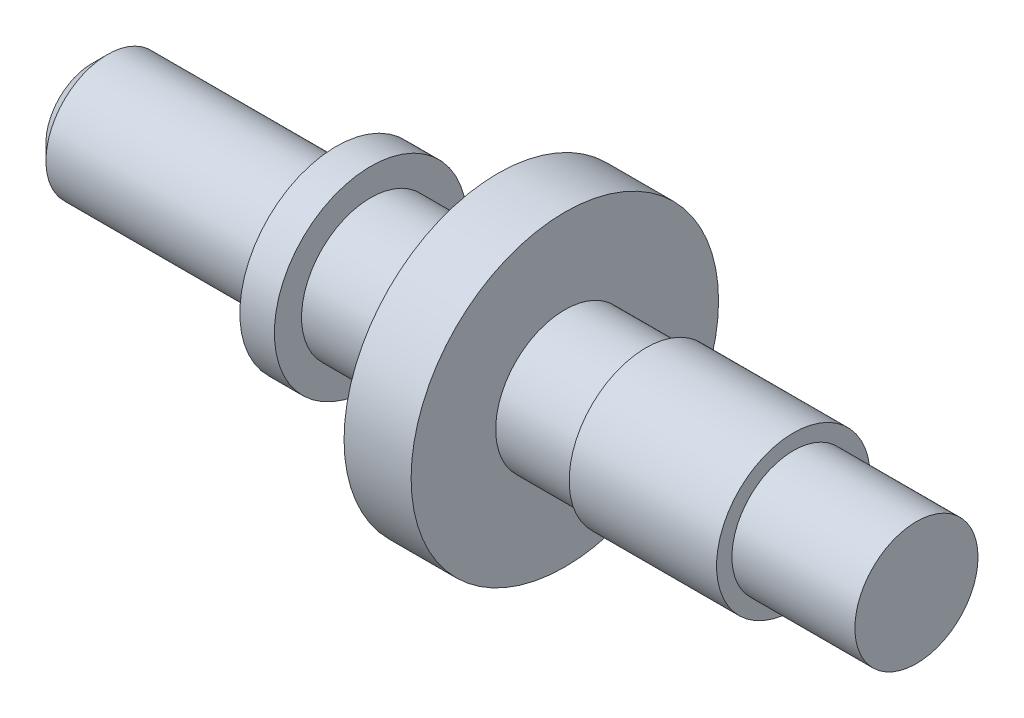
SolidWorks part; units mm, degrees
ref_plane "Front Plane" through (0, 0, 0) normal (0, 0, 1) x (1, 0, 0)
ref_plane "Top Plane" through (0, 0, 0) normal (0, 1, 0) x (1, 0, 0)
ref_plane "Right Plane" through (0, 0, 0) normal (1, 0, 0) x (0, 0, -1)
sketch "Model" plane through (0, 0, 0) normal (0, 0, 1) x (1, 0, 0)
  line L0 (49.5133, -13.474) -> (49.5171, -14.4694)
  line L1 (22.0151, -12.2049) -> (22.0151, -13.974)
  line L2 (57.5171, -18.474) -> (57.5171, -14.4694)
  line L3 (57.5171, -14.4694) -> (49.5171, -14.4694)
  line L4 (49.5133, -13.474) -> (39.9239, -13.474)
  line L5 (39.9239, -13.474) -> (39.9239, -13.974)
  line L6 (39.9239, -13.974) -> (34.6431, -13.974)
  line L7 (34.6431, -13.974) -> (34.6431, -8.474)
  line L8 (34.6431, -8.474) -> (30.2807, -8.474)
  line L9 (30.2807, -8.474) -> (30.2807, -13.974)
  line L10 (30.2807, -13.974) -> (22.0151, -13.974)
  line L11 (22.0151, -12.2049) -> (19.769, -12.2049)
  line L12 (19.769, -12.2049) -> (19.769, -14.474)
  line L13 (19.769, -14.474) -> (11.769, -14.474)
  line L14 (11.769, -14.474) -> (4.8845, -14.474)
  line L15 (4.8845, -14.474) -> (3.8845, -15.474)
  line L16 (3.8845, -15.474) -> (3.8845, -18.474)
  line L17 (3.8845, -18.474) -> (57.5171, -18.474)
  line L18 (3.8845, -18.474) -> (-2.2977, -18.474) construction
revolve "Revolve1" add sketch "Model" angle 360 about L18
